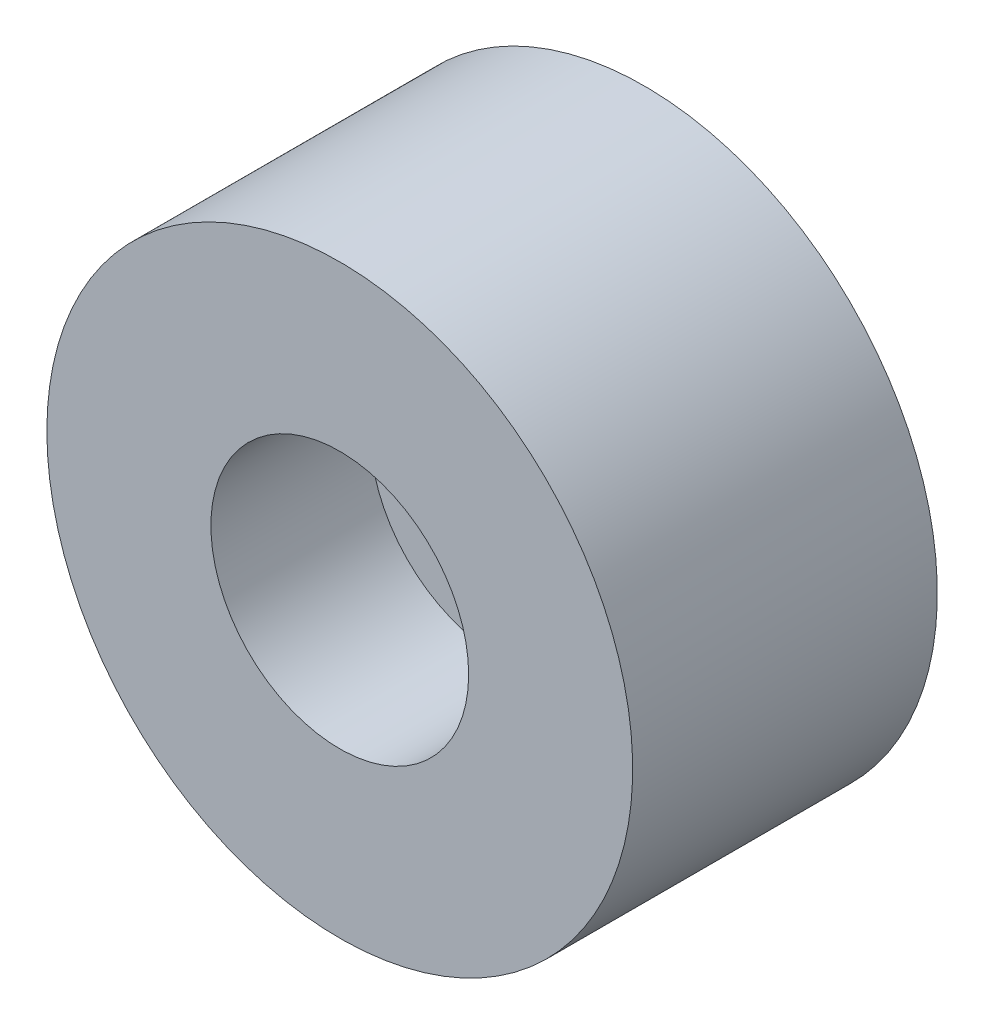
from build123d import *

# Parameters (mm, degrees)
SKETCH_1_R                   = 12.5
EXTRUDE_1_DEPTH              = 13
HOLE_WIZARD_M6_1_D           = 6.6
HOLE_WIZARD_M6_1_CBORE_D     = 11
HOLE_WIZARD_M6_1_CBORE_DEPTH = 6.8


with BuildPart() as part:
    # 草图1 → 凸台-拉伸1 (new body)
    with BuildSketch(Plane.XY):
        with Locations(Location((0, 0, 0), (0, 0, 180))):
            Circle(SKETCH_1_R)
    extrude(amount=EXTRUDE_1_DEPTH)

    # M6 六角圆柱头螺钉的柱形沉头孔1 (through all)
    with Locations(Plane.XY.offset(13)):
        with Locations((0, 0)):
            CounterBoreHole(HOLE_WIZARD_M6_1_D / 2, HOLE_WIZARD_M6_1_CBORE_D / 2, HOLE_WIZARD_M6_1_CBORE_DEPTH)


solid = part.part
